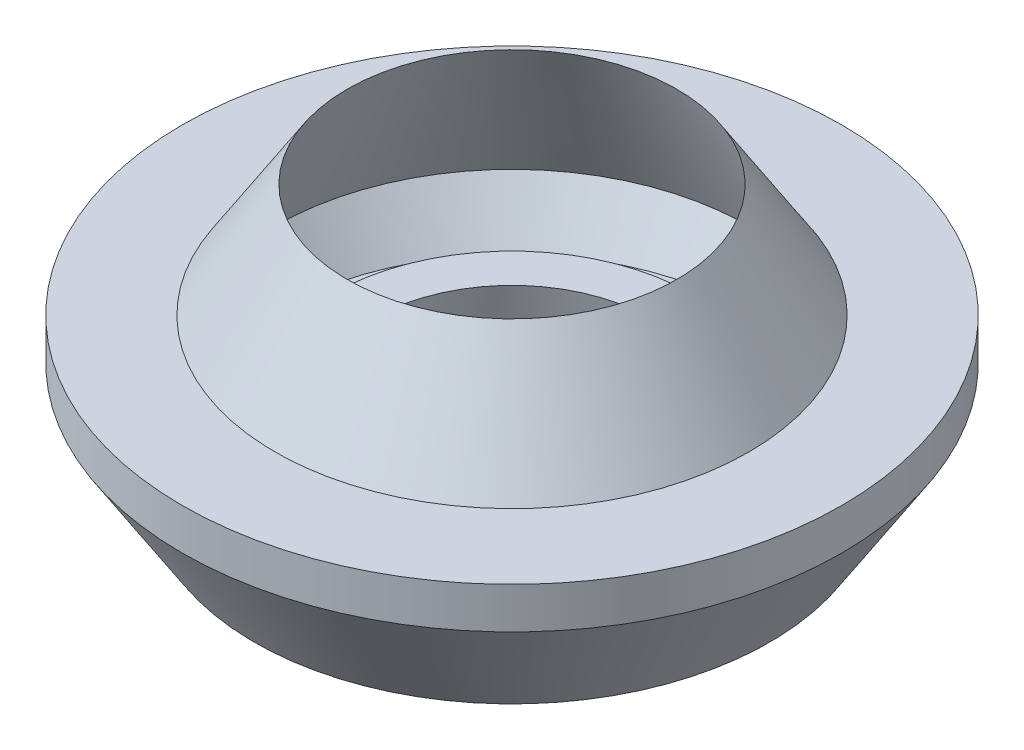
SolidWorks part; units mm, degrees
material "橡胶"
ref_plane "前视基准面" through (0, 0, 0) normal (0, 0, 1) x (1, 0, 0)
ref_plane "上视基准面" through (0, 0, 0) normal (0, 1, 0) x (1, 0, 0)
ref_plane "右视基准面" through (0, 0, 0) normal (1, 0, 0) x (0, 0, -1)
sketch "草图1" plane through (0, 0, 0) normal (0, 0, 1) x (1, 0, 0)
  line L0 (0, 12.9153) -> (0, -11.3198) construction
  line L1 (-18.6998, 0) -> (8.8958, 0) construction
  line L2 (16, 26) -> (23, 15)
  line L3 (23, 15) -> (32, 15)
  line L4 (32, 15) -> (32, 11)
  line L5 (32, 11) -> (25, 0)
  line L6 (25, 0) -> (15, 0)
  line L7 (15, 0) -> (13.45, 8)
  line L8 (13.45, 8) -> (17.5244, 8)
  line L9 (17.5244, 8) -> (18.2994, 4)
  line L10 (18.2994, 4) -> (22.8042, 4)
  line L11 (22.8042, 4) -> (27.2588, 11)
  line L12 (27.2588, 11) -> (22.9946, 11)
  line L13 (22.9946, 11) -> (16, 26)
  dimension "D1" = 4
  dimension "D2" = 4
  dimension "D3" = 4
  dimension "D4" = 4
  dimension "D5" = 25
  dimension "D6" = 15
  dimension "D7" = 26
  dimension "D8" = 64
  dimension "D9" = 46
  dimension "D10" = 32
  dimension "D11" = 50
  dimension "D12" = 30
  dimension "D13" = 26.9
  dimension "D14" = 8
revolve "旋转1" add sketch "草图1" angle 360 about L0
